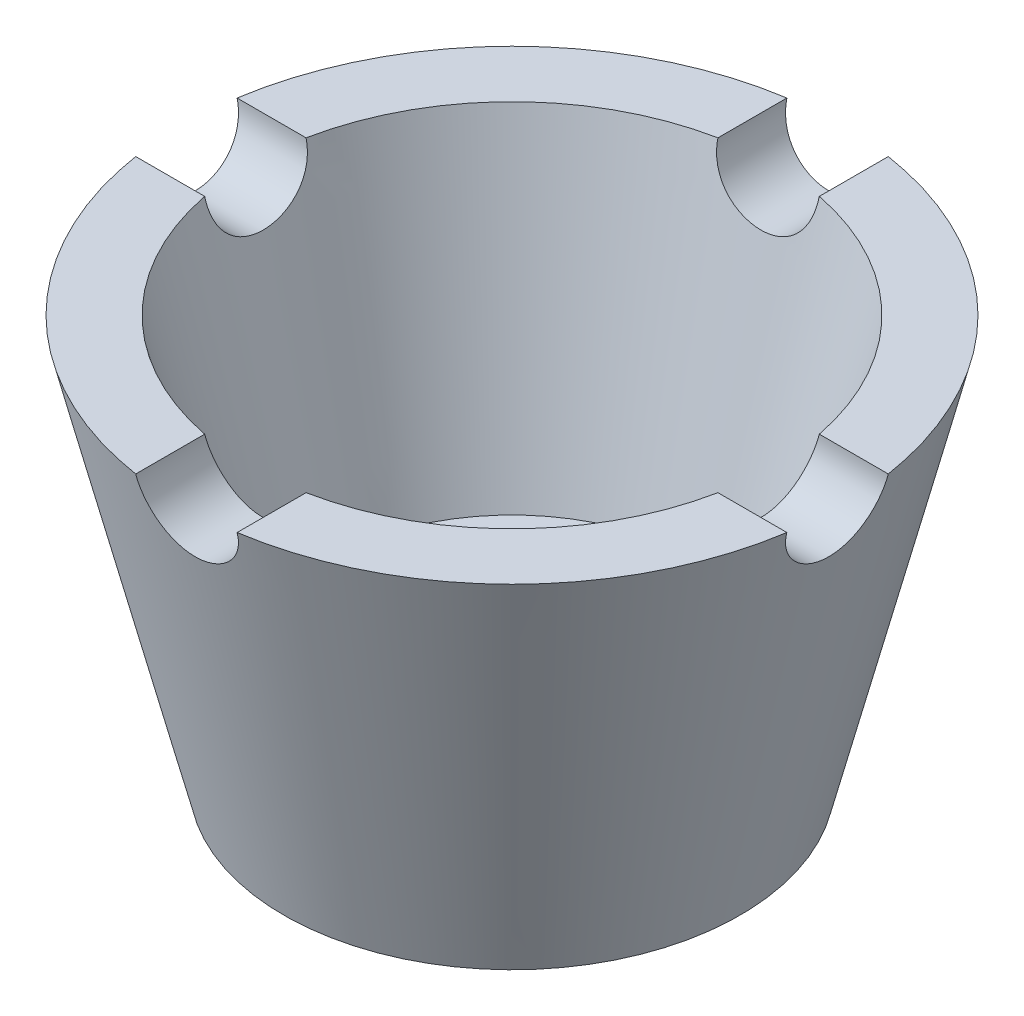
from build123d import *

# Parameters (mm, degrees)
SKETCH2_R          = 12.5
CUT_EXTRUDE1_DEPTH = 10
CUT_EXTRUDE2_DEPTH = 40
CIRPATTERN1_COUNT  = 4


with BuildPart() as part:
    # Sketch1 → Revolve1 (revolve)
    with BuildSketch(Plane.XY, mode=Mode.PRIVATE) as revolve1_sk:
        Polygon((32.5, 20), (22.5, -20), (0, -20), (0, -10), (18.299953358, -10), (25.799953358, 20), align=None)
    revolve(revolve1_sk.sketch.rotate(Axis((0, 20, 0), (0, -1, 0)), 180), axis=Axis((0, 20, 0), (0, -1, 0)))

    # Sketch2 → Cut-Extrude1 (cut)
    with BuildSketch(Plane(origin=(0, -10, 0), x_dir=(1, 0, 0), z_dir=(0, 1, 0))):
        with Locations(Location((0, 0, 0), (0, 0, 180))):
            Circle(SKETCH2_R)
    extrude(amount=-CUT_EXTRUDE1_DEPTH, mode=Mode.SUBTRACT)

    # Sketch4 → Cut-Extrude2 (cut, symmetric)
    with BuildSketch(Plane.XY):
        with BuildLine():
            Line((-5, 20), (5, 20))
            ThreePointArc((5, 20), (0, 15), (-5, 20))
        make_face()
    cut_extrude2 = extrude(amount=CUT_EXTRUDE2_DEPTH, both=True, mode=Mode.SUBTRACT)

    # CirPattern1: Cut-Extrude2 ×4 about axis
    cirpattern1_axis = Axis((0, -20, 0), (0, 1, 0))
    for i in range(1, CIRPATTERN1_COUNT):
        add(cut_extrude2.rotate(cirpattern1_axis, i * 360 / CIRPATTERN1_COUNT), mode=Mode.SUBTRACT)


solid = part.part
